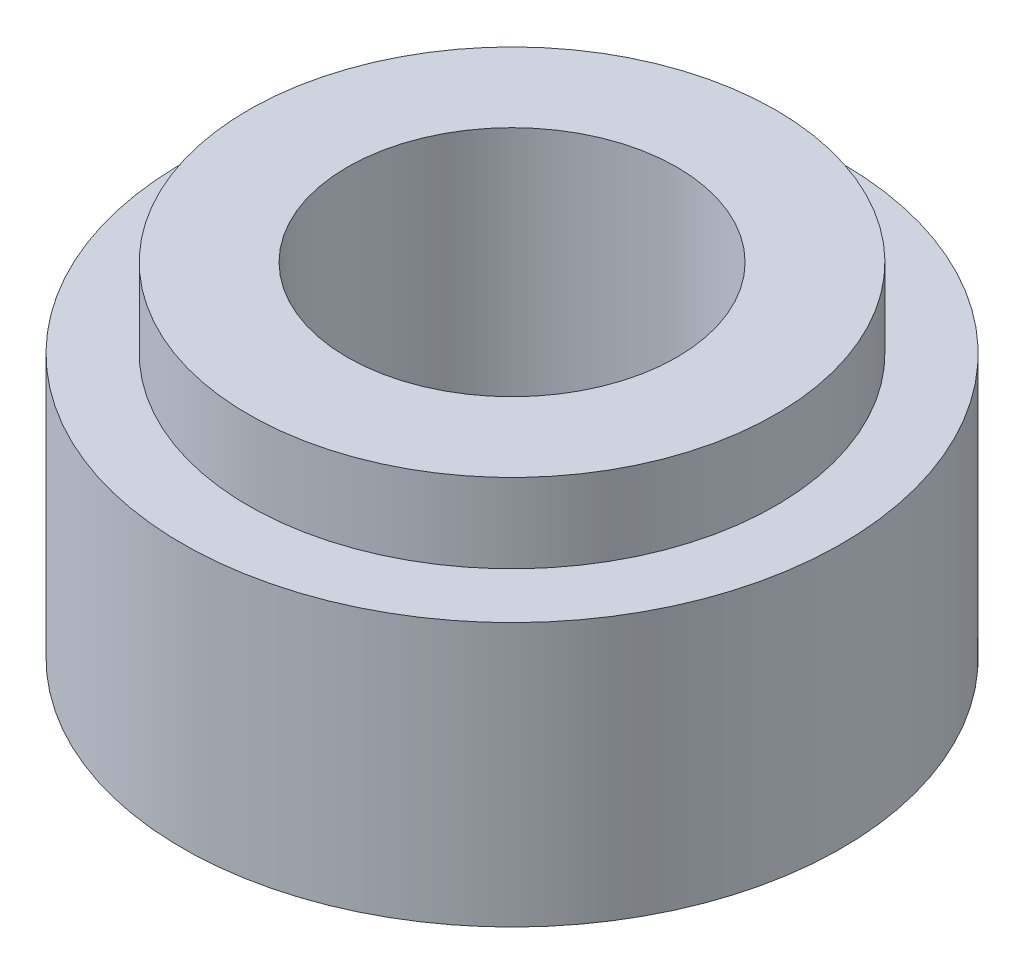
SolidWorks part; units mm, degrees
material "45"
ref_plane "Front Plane" through (0, 0, 0) normal (0, 0, 1) x (1, 0, 0)
ref_plane "Top Plane" through (0, 0, 0) normal (0, 1, 0) x (1, 0, 0)
ref_plane "Right Plane" through (0, 0, 0) normal (1, 0, 0) x (0, 0, -1)
sketch "Sketch1" plane through (0, 0, 0) normal (0, 0, 1) x (1, 0, 0)
  line L0 (0, 0) -> (0, 18.7288) construction
  line L1 (0, 0) -> (12.5, 0)
  line L2 (12.5, 0) -> (12.5, 10)
  line L3 (12.5, 10) -> (10, 10)
  line L4 (10, 10) -> (10, 13)
  line L5 (10, 13) -> (0, 13)
  line L6 (0, 0) -> (0, 13)
  dimension "D1" = 25
  dimension "D2" = 20
  dimension "D3" = 10
  dimension "D4" = 13
revolve "Revolve1" add sketch "Sketch1" angle 360 about L0
hole_wizard "M14x1.5 Tapped Hole1" positions "Sketch2" profile "Sketch3" tap size "M14x1.5" standard "GB"
sketch "Sketch2" plane through (0, 0, 0) normal (0, -1, 0) x (-1, 0, 0)
  point P0 (0, 0)
sketch "Sketch3" plane through (0, 0, 0) normal (1, 0, 0) x (0, 0, -1)
  line L0 (0, 0) -> (0, 39.2554)
  line L1 (0, 39.2554) -> (6.25, 35.5)
  line L2 (6.25, 35.5) -> (6.25, 0)
  line L5 (6.25, 0) -> (0, 0)
  line L10 (0, 39.2554) -> (-6.25, 35.5) construction
  line L11 (0, -6.35) -> (0, 107.95) construction
  dimension "螺纹孔钻头直径" = 12.5
  dimension "螺纹孔钻头深度" = 35.5
  dimension "导头角度" = 118
cosmetic thread "Cosmetic thread1" parameters "D1"=28, "D2"=14
